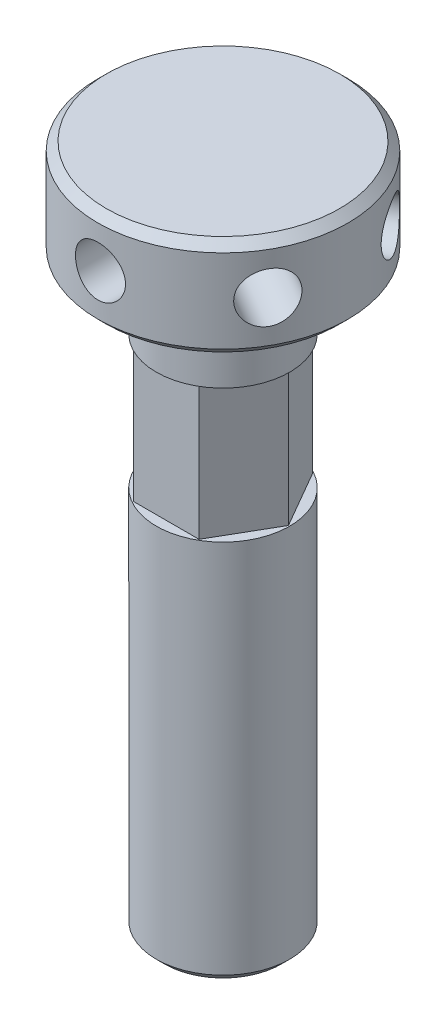
from build123d import *

# Parameters (mm, degrees)
SKETCH1_R           = 4
BOSS_EXTRUDE1_DEPTH = 35
SKETCH2_R           = 7.5
BOSS_EXTRUDE2_DEPTH = 6
CHAMFER1_SIZE       = 0.5
SKETCH3_R           = 1.5
CUT_EXTRUDE1_DEPTH  = 9.5
CIRPATTERN1_COUNT   = 6
SKETCH5_W           = 1.2
SKETCH5_H           = 8
CUT_EXTRUDE3_DEPTH  = 5
CIRPATTERN3_COUNT   = 6


with BuildPart() as part:
    # Sketch1 → Boss-Extrude1 (new body)
    with BuildSketch(Plane(origin=(0, 0, 0), x_dir=(1, 0, 0), z_dir=(0, 1, 0))):
        with Locations(Location((0, 0, 0), (0, 0, 270))):
            Circle(SKETCH1_R)
    extrude(amount=BOSS_EXTRUDE1_DEPTH)

    # Sketch2 → Boss-Extrude2 (add)
    with BuildSketch(Plane(origin=(0, 35, 0), x_dir=(1, 0, 0), z_dir=(0, 1, 0))):
        with Locations(Location((0, 0, 0), (0, 0, 270))):
            Circle(SKETCH2_R)
    extrude(amount=BOSS_EXTRUDE2_DEPTH)

    # Chamfer1
    chamfer1_edges = [part.edges().sort_by_distance(p)[0] for p in [
        (0, 0, -4),
        (0, 35, -7.5),
        (0, 41, -7.5),
    ]]
    chamfer(chamfer1_edges, length=CHAMFER1_SIZE)

    # Sketch3 → Cut-Extrude1 (cut, symmetric)
    with BuildSketch(Plane.XY):
        with Locations(Location((0, 38, 0), (0, 0, 90.000000044))):
            Circle(SKETCH3_R)
    cut_extrude1 = extrude(amount=CUT_EXTRUDE1_DEPTH, both=True, mode=Mode.SUBTRACT)

    # CirPattern1: Cut-Extrude1 ×6 about axis
    cirpattern1_axis = Axis((0, 41, 0), (0, -1, 0))
    for i in range(1, CIRPATTERN1_COUNT):
        add(cut_extrude1.rotate(cirpattern1_axis, i * 360 / CIRPATTERN1_COUNT), mode=Mode.SUBTRACT)

    # Sketch5 → Cut-Extrude3 (cut, symmetric)
    with BuildSketch(Plane(origin=(0, 0, 0), x_dir=(0, 0, -1), z_dir=(1, 0, 0))):
        with Locations((4, 27)):
            Rectangle(SKETCH5_W, SKETCH5_H)
    cut_extrude3 = extrude(amount=CUT_EXTRUDE3_DEPTH, both=True, mode=Mode.SUBTRACT)

    # CirPattern3: Cut-Extrude3 ×6 about axis
    cirpattern3_axis = Axis((0, 0, 0), (0, 1, 0))
    for i in range(1, CIRPATTERN3_COUNT):
        add(cut_extrude3.rotate(cirpattern3_axis, i * 360 / CIRPATTERN3_COUNT), mode=Mode.SUBTRACT)


solid = part.part
